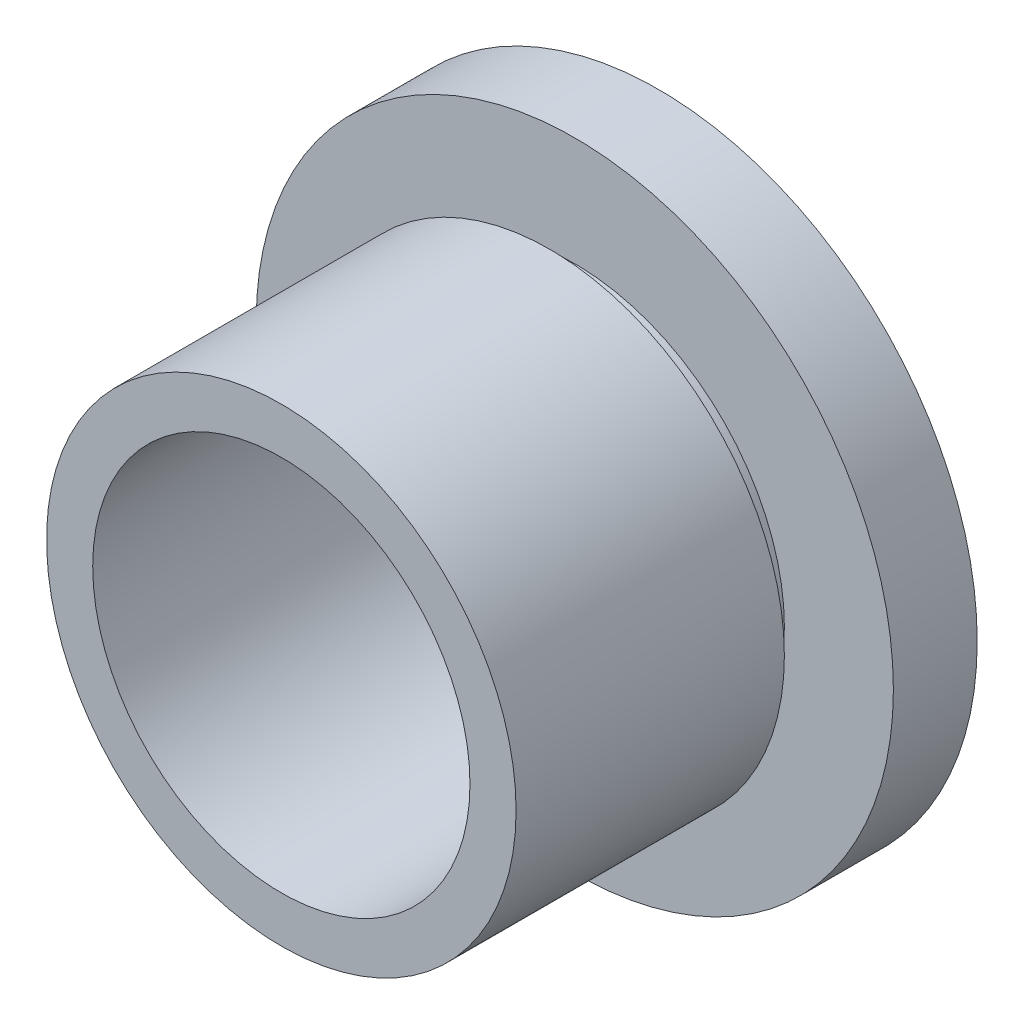
SolidWorks part; units mm, degrees
ref_plane "Front Plane" through (0, 0, 0) normal (0, 0, 1) x (1, 0, 0)
ref_plane "Top Plane" through (0, 0, 0) normal (0, 1, 0) x (1, 0, 0)
ref_plane "Right Plane" through (0, 0, 0) normal (1, 0, 0) x (0, 0, -1)
other "Configuration Table"
sketch "Sketch1" plane through (0, 0, 0) normal (1, 0, 0) x (0, 0, -1)
  line L0 (-12.0113, 0) -> (11.2921, 0) construction
  line L1 (0, 22.5) -> (0, 28)
  line L2 (0, 28) -> (32, 28)
  line L3 (32, 28) -> (32, 25)
  line L4 (32, 25) -> (35, 25)
  line L5 (35, 25) -> (35, 38)
  line L6 (35, 38) -> (45, 38)
  line L7 (45, 38) -> (45, 17.5)
  line L8 (35, 17.5) -> (35, 22.5)
  line L9 (35, 22.5) -> (0, 22.5)
  line L10 (35, 17.5) -> (45, 17.5)
  dimension "D1" = 45
  dimension "D2" = 56
  dimension "D3" = 76
  dimension "D4" = 35
  dimension "D5" = 10
  dimension "D6" = 10
  dimension "D7" = 45
  dimension "D8" = 3
  dimension "D9" = 3
revolve "Revolve1" add sketch "Sketch1" angle 360 about L0
cosmetic thread "Cosmetic Thread1"
cosmetic thread "Cosmetic Thread2"
